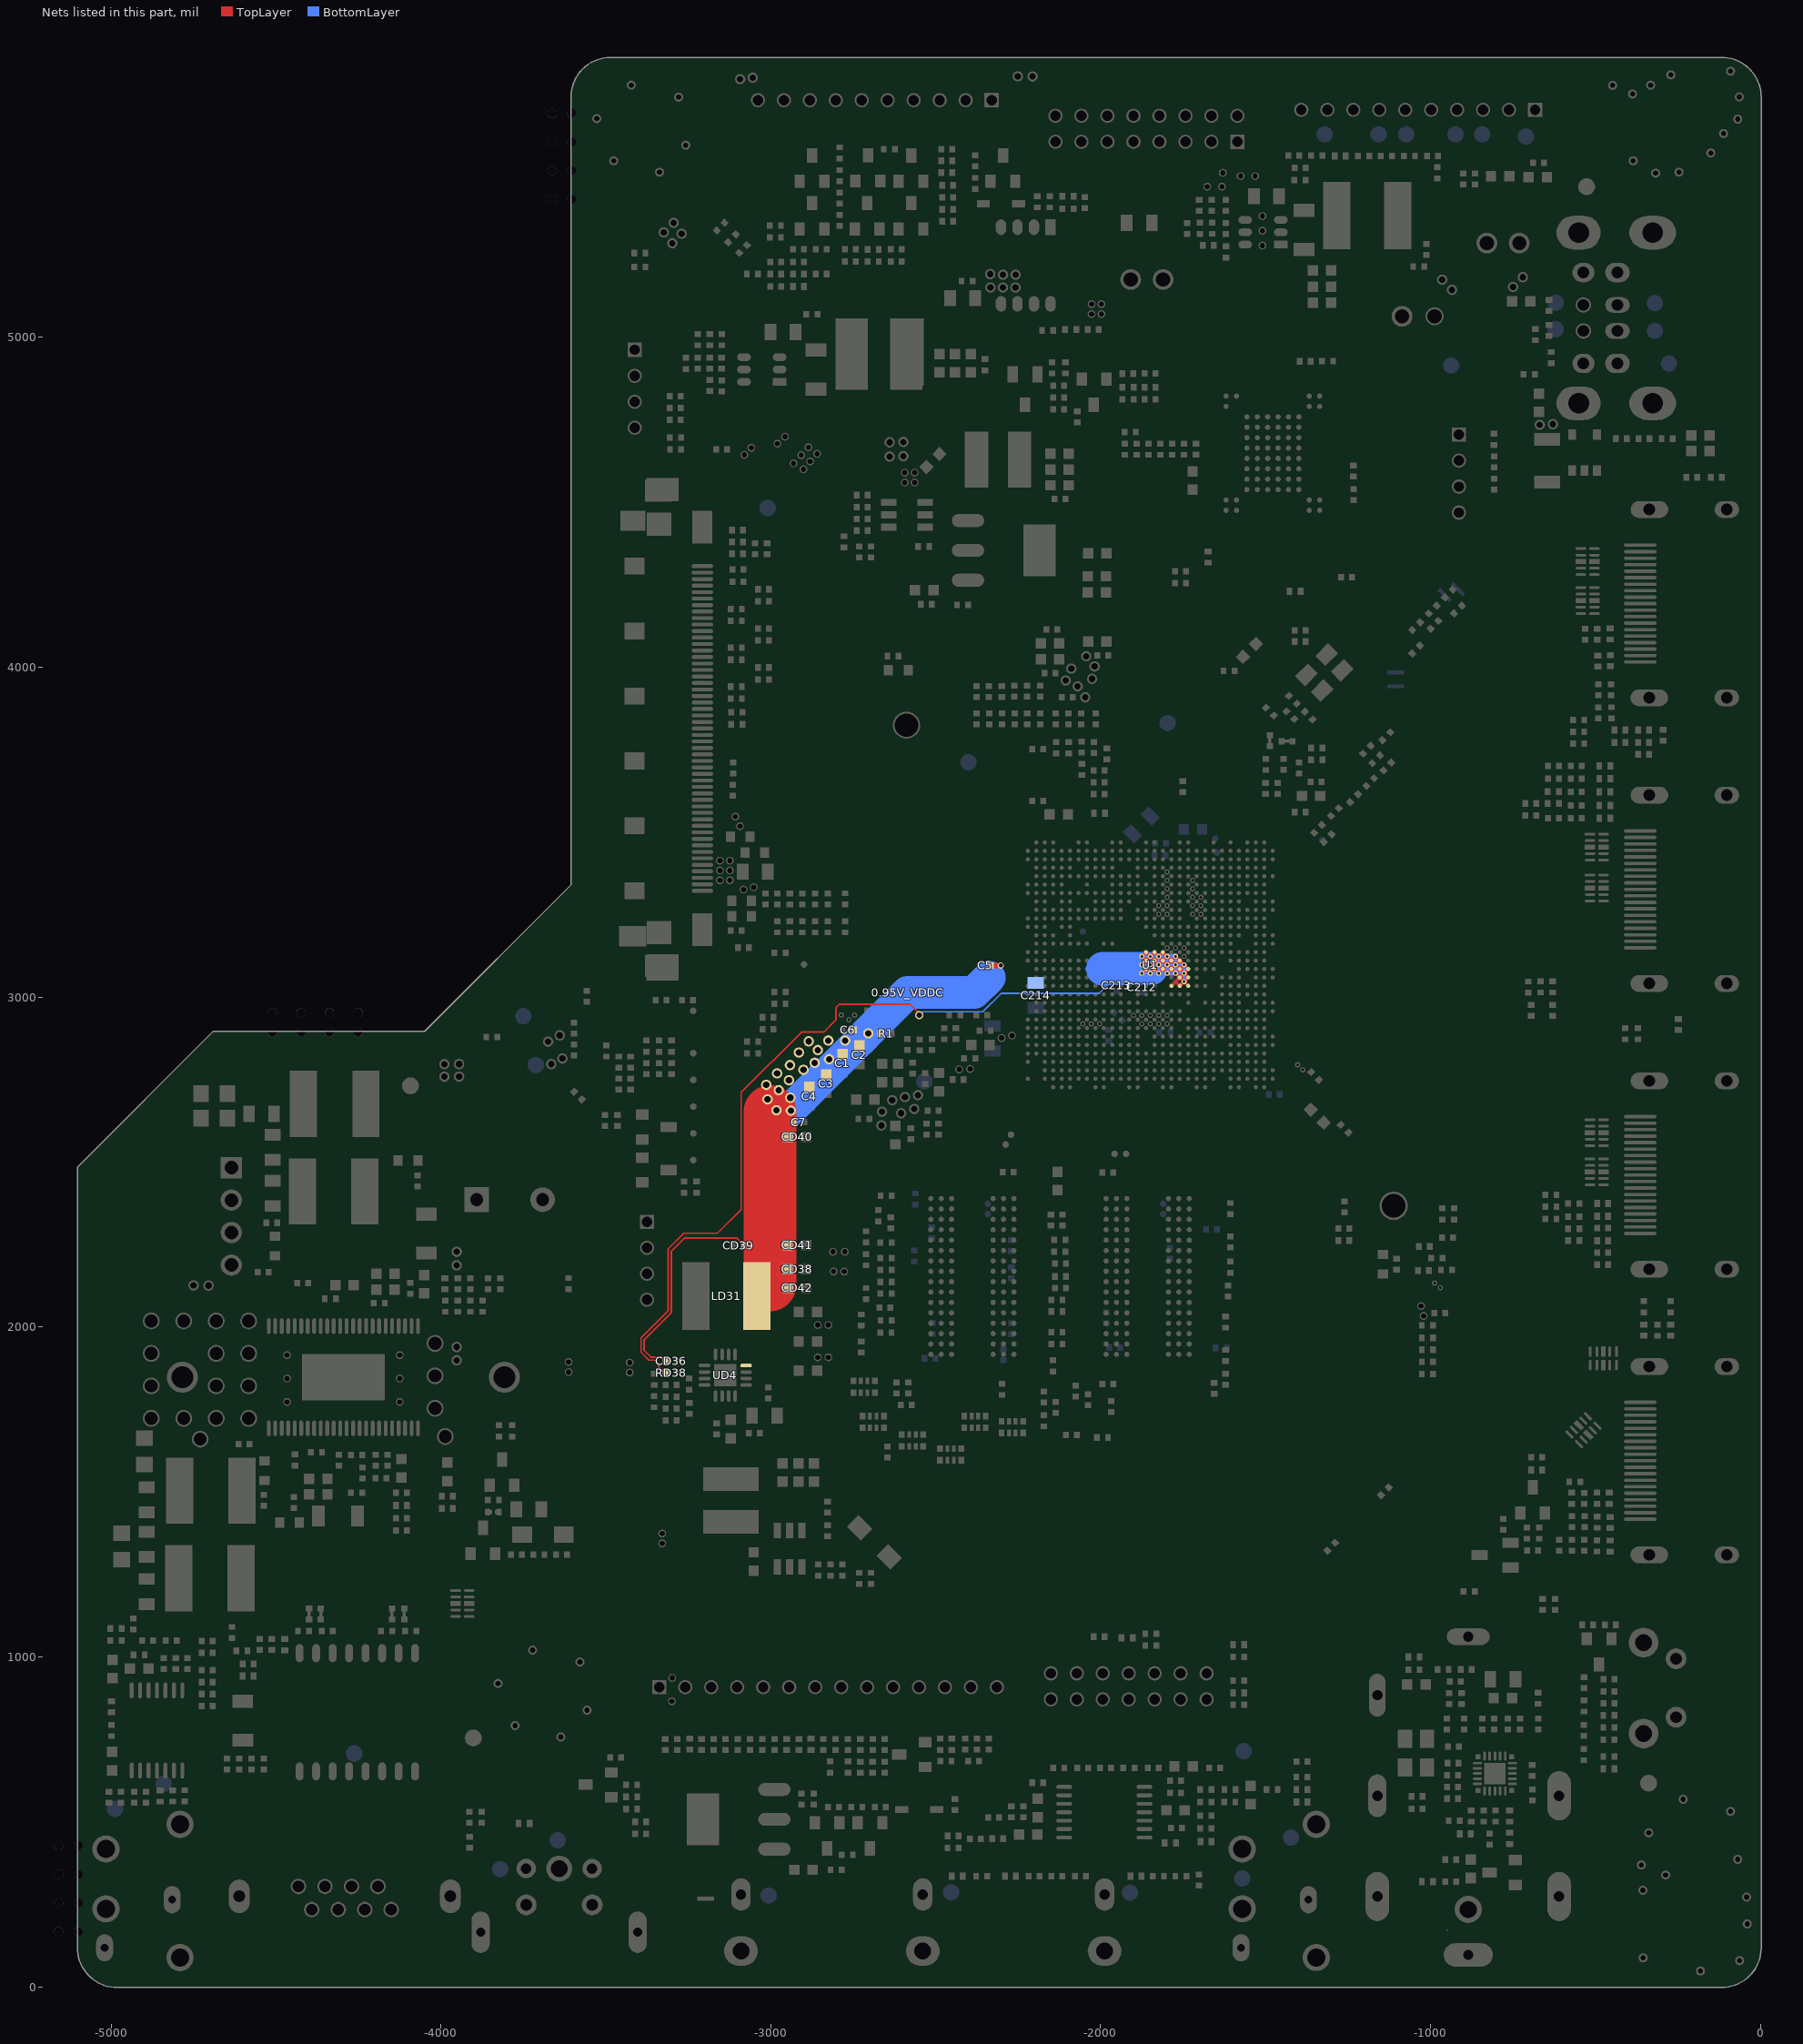
[diagram p0: the nets of this part, all layers, seen from the top]
# Altium PCB MISC86290.PcbDoc (part 7 of 31)
Units mil, origin at the board's own origin, x right, y up, seen from the top; angles counter-clockwise.
Board outline 5104.71 x 5851.49 mil, 2 copper layers (TopLayer, BottomLayer), stack 61.855 mil thick; 1026 components, 667 nets, 4280 pads, 2294 vias.

## Part data (continued)
CA30 CA31: library part 004.003.0000956-D, "Ceramic capacitor,CAP MC,50V,10uF,±10%,X5R,1206,SMD,TP-D"
CA32 CA33 CA34 CA35 CO2: library part 330pF-0402-NPO-±5%-50V-D
CA53 CA56 CO15 CO16: library part 220pF-0402-NPO-±5%-50V-D
CD1 CD13: library part 10uF-1206-X5R-±10%-16V-D
CD2 CD5 CD7 CD32 CD39 CP2 CT10 CT15 CT16 CT17 CT27 CT32 CU14: library part 0.1uF-0402-Y5V-+80%-20%-16V-D
CD6: library part 10pF-0402-NPO-±5%-50V-D
CD15: library part 8pF-0402-NPO-±5%-50V-D
CD23 CD53: library part 004.003.0000527-D, "Ceramic capacitor,CAP MC,50V,18pF,±5%,NPO,0402,SMD,TP-D"
CD34 CM2 CM4 CM16: library part 0.022uF-0402-X7R-±10%-16V-D
CD36 CT24: library part 120pF-0402-NPO-±5%-50V-D
CE1 CE2 CE3 CE4: library part 7pF-0402-NPO-±5%-50V-D
CE5: library part 1000pF-1206-X7R-±20%-2000V-D
CE8: library part 0.01uF-0402-X7R-±10%-16V-D
CH1 CH2 CH4 CH5 CH6 CH11 CH12 CH13 CH14 CH21 CH22 CH23 CH24 CH31 CH32 CH33 CH34: library part 5pF-0402-NPO-±5%-50V-D
CH7: library part 2.2uF-0402-X5R-±20%-6.3V-D
CH15 CH16 CH17 CH18 CK1 CT26: library part 22pF-0402-NPO-±5%-50V-D
CI1 CI3 CI5 CT6 CT7 CT8 CT12 CT14 CT21: library part 56pF-0402-NPO-±5%-50V-D
CI4 CI6: library part 1uF-0402-X5R-±20%-16V-D
CK7 CK8 CM1 CO11 CO12 CO31 CO32 CT1 CT2 CT19 CT20: library part 1000pF-0402-X7R-±10%-50V-D
CM3 CU15 CU16: library part 22uF-0603-X5R-±20%-6.3V-D
CM15 CO18 CO42 CU4 CU11 CU12 CU13: library part 0.1uF-0402-X7R-±10%-16V-D
CN1 CN2 CN3: library part 4PIN-2.0-D-H-G-LD-DHMI
CN16: library part XXX.XXX.0000613-DHMI, "Connector socket,connect jack,10Pin,D2.0,D,L=2.8mm,DIP,CNJST-DHMI"
CN17: library part XXX.XXX.0000646-DHMI, "Connector socket,connect jack,10Pin,D2.0,D,SNAP,L=2.8mm,DIP,CNJST-DHMI"
CN19: library part 10PIN-2.0-D-H-G-带扣-J-DHMI
CNA3: library part XXX.XXX.0000762-DLMI, "Connector socket,connect jack,4Pin,D2.50,L,STEP,Beige,L=2.8mm,DIP,CNJST-DLMI"
CNA4: library part XXX.XXX.0001836-DLMI, "Connector socket,connect jack,4PIN,D2.50,L,SNAP,STEP,Fool-proofing,Nature,L=3.0mm,DIP,AMA-DLMI"
CNA5: library part XXX.XXX.0002239-DHMI, "Gold-plated pin,pin connector,2×7Pin,D,D2.0,L=2.6mm,DIP,LD-DHMI"
CNK2: library part 14PIN-2.0-D-H-G-DHMI-IR&KEY
CNK3: library part 14PIN-2.0-D-H-G-带扣-J-DHMI
CNP2: library part 2×8PIN-2.0-D-H-G-带扣-J-DHMI, "CN-keyed"
CNW1: library part XXX.XXX.0002122, "FPC socket,FPC connector (B),51Pin,D0.5,L,Bottom,lock,SMD,DEREN-D"
CNW2: library part 51PIN-0.5-L-M-下接-翻盖-H=2.7mm-XFE-D, "CN-FFC socket-flip lid"
CNW3: library part PKG-003664/P000081334, "FFC socket,FFC connector,51Pin,D0.5,Bottom,lock,SMD,F05035FA51M1WL,CT-D"
CNW12: library part FI-RE51S-HF-J-R1500-D, "CN-FFC socket-bottom contact"
CO20 CO36: library part 10uF-0603-X5R-±20%-6.3
CO26 CO27: library part 004.003.0000501-D, "Ceramic capacitor,CAP MC,50V,100pF,±5%,NPO,0402,SMD,TP-D"
CT3: library part 10uF-0603-X5R-±20%-10V-D
CT4 CT5: library part 27pF-0402-NPO-±5%-50V-D
CT9 CT23: library part 30pF-0402-NPO-±5%-50V-D
CT25: library part 47pF-0402-NPO-±5%-50V-D
CT28: library part 0.1uF-0805-X7R-±10%-50V-D, "CAP"
CT39 CT40: library part 18pF-0402-NPO-±5%-50V-D
D4 D5 D40 D41 DA1 DA2 DA5 DA6 DG1 DG11 DH15 DI1 DI2 DI3 DK9 DK10 DO1 DO2 DO11 DO12 DO31 DO32 DR1 DR2 DR4 DR5 DT2 DT3: library part AVLC18S02003-D
DA9: library part PMLL4148L-F-D
DD2: library part 5.6V-LL-34-1/2W-D
DE1 DE2 DF5 DF6 DU1 DU2 DW1 DW2: library part AIES12U020R2-D
DH1 DH2 DH3 DH4 DH5 DH11 DH12 DH13 DH14 DH21 DH22 DH23 DH24 DH31 DH32 DH33 DH34 DH35 DH36 DH37: library part "TVS管,DIO ESD,0.4pF,11V,SOD882,SMD,PESD5V0F1BL,NXP-D"
DM11 DR3: library part 1N4148WS-D
DT1: library part BAV99-BR-D
EA1: library part 004.003.0000454-DHMI, "Aluminium electrolytic capacitor,CAP AL,35V,470uF,±20%,RK,P,5.0mm,10×13,DIP,TP,XL-DHMI"
ED1 ED11: library part 470uF-10V-±20%-6.3×11-105℃-黑底白字-编带-F=2.5-XF-DHAI, "Electrolytic"
EP1: library part 004.003.0000158-DHAI, "Aluminium electrolytic capacitor,CAP AL,16V,220uF,±20%,LD,KF,P,2.5mm,6.3×11,DIP,TP,CapXon-DHAI"
FT1 LA10 LA12 RT4: library part FCM1005KF-121T06(120ohm-500mA)-D
FU1: library part NSMD110(1206-1.1A)-D
H1 H2 H3 H4 H5 H6: library part "Location hole-D"
HS1: library part 004.040.0000611-HS, "Heat sink,aluminium alloy,55.0×55.0×10.0mm,black,anodized,THD-HS"
HSA1: library part 27*10*10-HS, "HS-natural colour"
LA1 LA2 LA3 LA4: library part MPIT6045-150M-LF-D
LD1 LD3 LD4: library part SWPA6045S4R7MT-D
LD2: library part MGSD54-6R8M-LF-D
LD21 LD51: library part SLN43T-6R8M-D
LD31: library part 004.004.0000652-D, "Power inductor,Power Inductor,2.2uH,±20%,4.60A,DR6.0×4.5,SMD,MPIT6045-2R2M-LF,Microgate-D"
LF1: library part HCB1005KF-121T20(120ohm-1200mA)-D
LO1 R1 R3 R130 R135 R136 R137 R171 RD3 RD4 RD13 RD14 RD30 RD51 RE6 RF3 RF4 RF5 RF6 RF7 RF8 RG41 RG42 RG43 RG44 RI115 RO3 RO51 RO52 RR18 RT1 RT3 RT7 RT40 RU13 RU14 RU15 RU16 RU17 RW10 RW11 RW389 RW393 RW395: library part 0ohm-0402-±5%-1/16W-D
LO2 LO3: library part 004.004.0000326-D, "Ferrite bead,BEAD,120ohm,0402,500mA,SMD,TP,FCM1005KF-121T06,Tai-tech-D"
LT3 LT4 LT5 LT6 LT7 LT9: library part SDCL1005CR33JTDF-D
LT10: library part 680ohm-0402-±5%-1/16W-D
LU11: library part HCB1608KF-121T20(120ohm-2000mA)-D
M1 M2 M3 M4 M5 M6: library part MARK-D
MAC: library part Barcode
NC/ESD: library part ESD-T
P1(用于U1上): library part 0.05g-导热硅脂, "Thermal grease"
QA2: library part 3CG3906M-D, "Q-PNP-#-#-#"
QA3 QG1 QG2 QG11 QG12 QG30 QG31 QK1 QO21 QR3: library part LMBT3904LT1G-D-NPN, "Q-NPN-#-#-#"
QM1: library part WPM3407C-3/TR-D
QM2: library part AO4459-D
QM4 QM11 QR4: library part KMBT3904-D
QR1 QR2: library part LMBT3906LT1G-D-PNP
QW1 QW2: library part 004.007.0000056-D, "MOSFET,NMOS,0.3A,60V,3.3ohm@ID=0.3A@VGS=4.5V,SOT-23,ME2N7002E,MATSUKI-D"
R4 R5 R6 R7 R8 R9 R10 R11 R12 R13 R14 R15 R16 R17 R18 R19 R20 R21 R22 R23 R24 R25 R26 R27 RD21 RD24 RD52: library part 004.002.0000689-D, "Thick-film resistor,RES,1/16W,4.7Kohm,±5%,0402,SMD-D"
R30 R31 R138 R139 R151 R152 R153 RA11 RA20 RG2 RG30 RG31 RK1 RK28 RK30 RM1 RM2 RM11 RM13 RM15 RO20 RO22 RO23 RO26 RO27 RO28 RO29 RO30 RO43 RO44 RO45 RO46 RO47 RP5 RR3 RR9 RR13 RR15 RR16 RT5 RT6 RU3 RU6 RU11 RU12 RU18 RW4 RW251 RW252 RW405 RW406 RW407 RW408 RW409 RW410 RW412 RW413 RW414 RW415 RW416 RW417: library part 4K7ohm-0402-±5%-1/16W-D
R39: library part 004.002.0000721-D, "Thick-film resistor,RES,1/16W,68ohm,±5%,0402,SMD-D"
R41 R54 R55 R58 R59 R60 R61: library part 004.002.0000728-D, "Thick-film resistor,RES,1/16W,75ohm,±5%,0402,SMD-D"
R42 R208 RD2: library part 1Mohm-0402-±5%-1/16W-D
R44 R120 RF1: library part 004.002.0000572-D, "Thick-film resistor,RES,1/16W,1Kohm,±5%,0402,SMD-D"
R45 R62 R63 R107 R108 R121 R123: library part 004.002.0000577-D, "Thick-film resistor,RES,1/16W,10Kohm,±5%,0402,SMD-D"
R46 R47: library part 004.002.0000583-D, "Thick-film resistor,RES,1/16W,11Kohm,±1%,0402,SMD-D"
R48 R49 R64 R100: library part 004.002.0000636-D, "Thick-film resistor,RES,1/16W,240ohm,±1%,0402,SMD-D"
R50 R51 R52 R53 R56 R57: library part 004.002.0000626-D, "Thick-film resistor,RES,1/16W,22ohm,±5%,0402,SMD-D"
R65 R66 R67 R101 R102 R103 R104 R118: library part 004.002.0000575-D, "Thick-film resistor,RES,1/16W,10Kohm,±1%,0402,SMD-D"
R72 R73 R140 R141 RA9 RH37 RH38 RR5 RR8 RT2 RT8 RT9 RW5: library part 100ohm-0402-±5%-1/16W-D
R105 R106: library part 004.002.0000447-D, "Thick-film resistor,RES,1/16W,56ohm,±1%,0402,SMD-D"
R122 R124: library part 004.002.0000630-D, "Thick-film resistor,RES,1/16W,2.2Kohm,±5%,0402,SMD-D"
R125 R126 R127 R128 R129 RH1 RH4 RH11 RH12 RH21 RH22 RH31 RH32: library part 004.002.0000658-D, "Thick-film resistor,RES,1/16W,33ohm,±5%,0402,SMD-D"
R143 R144 R145 R206 R207 RA21 RA23 RG1 RG7 RG12 RG17 RG37 RG38 RK2 RK10 RK26 RK33 RK42 RO24 RO25 RO39 RO40 RR1 RT10 RT12: library part 1Kohm-0402-±5%-1/16W-D
R146 R147 R148 R149 R150 RG3 RG13 RG39 RI1 RR10 RR11 RR14 RW26 RW73 RW421: library part 33ohm-0402-±5%-1/16W-D
R200 R201 R202 R203 R204 R205 RD1 RD11 RD12 RG32 RG33 RO13 RO14 RO33 RO34 RO55 RO56 RR19: library part 100Kohm-0402-±5%-1/16W-D
RA1 RA2 RA3 RA4 RH5 RH6 RH15 RH16 RH25 RH26 RH35 RH36 RK23: library part 22ohm-0402-±5%-1/16W-D
RA5 RA7 RA34 RG6 RG8 RG11 RG16 RG18 RG34 RG36 RH2 RH3 RH13 RH14 RH23 RH24 RH33 RH34 RI3 RI6 RK15 RM12 RP1 RR2 RR6 RR7 RR17 RU5 RU9 RU10 RW1 RW8 RW9: library part 10Kohm-0402-±5%-1/16W-D
RA6 RA8 RA12 RA14: library part 470ohm-0402-±5%-1/16W-D
RA15: library part 18Kohm-0402-±1%-1/16W-D
RA16 RA17 RA18 RA19: library part 18ohm-0603-±5%-1/10W-D
RA22: library part 8K2ohm-0402-±5%-1/16W-D
RA24 RA26 RK13 RO11 RO12 RO31 RO32: library part 33Kohm-0402-±5%-1/16W-D
RA30 RA31 RA32 RA33: library part 300ohm-2500mA-0805-D
RD5: library part 30Kohm-0402-±5%-1/16W-D
RD6: library part 3K3ohm-0402-±5%-1/16W-D
RD15 RD38: library part 60K4ohm-0402-±1%-1/16W-D
RD16: library part 10K5ohm-0402-±1%-1/16W-D
RD22 RD53 RD60: library part 004.002.0000718-D, "Thick-film resistor,RES,1/16W,6.2Kohm,±1%,0402,SMD-D"
RD23 RD54 RD55 RD57 RD59: library part 004.002.0000622-D, "Thick-film resistor,RES,1/16W,20Kohm,±1%,0402,SMD-D"
RD32 RD34 RD36: library part 113Kohm-0402-±1%-1/16W-D
RD33 RD35 RD37: library part 47Kohm-0402-±1%-1/16W-D
RD58: library part 004.002.0000558-D, "Thick-film resistor,RES,1/16W,0ohm,±5%,0402,SMD-D"
RE1 RE2 RE3 RE4: library part 75ohm-0402-±1%-1/16W-D
RE20 RE21 RE22 RE23 RT11 RT13: library part 0ohm-0402-PCB-D, "0ohm-0402-PCB-D"
RF2: library part 004.002.0000675-D, "Thick-film resistor,RES,1/16W,3.9Kohm,±1%,0402,SMD-D"
RF56: library part 004.002.0000757-D, "Thick-film resistor,RES,1/16W,120Kohm,±1%,0402,SMD-D"
RFT1: library part XXX.XXX.0002536, "RF shield can,RF SHLED,Single,H,F,T14.5,CH6.3,whole,25.0×14.5×10.0mm,DIP,LHD-DLMI"
RG4 RG5 RG14 RG15 RG35 RG40 RP8 RR4: library part 2K2ohm-0402-±5%-1/16W-D
RH17 RO1: library part 200ohm-0402-±5%-1/16W-D
RI2 RO2: library part 75ohm-0402-±5%-1/16W-D
RI4 RI5 RO19 RO21 RO41 RO42: library part 12Kohm-0402-±5%-1/16W-D
RI116 RO17 RO18 RO35 RO36: library part GND
RK14: library part 510ohm-0402-±5%-1/16W-D
RK24 RK34: library part 4K7ohm-0402-±1%-1/16W-D
RK27 RK32 RK35 RK36 RK37 RK38 RK40 RK41: library part 1K5ohm-0402-±5%-1/16W-D
RK29 RK31: library part 12Kohm-0402-±1%-1/16W-D
RM3 RM4 RM14 RO57 RO58: library part 47Kohm-0402-±5%-1/16W-D
RO15 RO16 RO37 RO38 RU1 RU2 RU7 RU8: library part 5R1ohm-0402-±5%-1/16W-D
RO53 RO54: library part 004.002.0000624-D, "Thick-film resistor,RES,1/16W,200Kohm,±5%,0402,SMD-D"
RP11 RP12 RP13 RP14 RP15 RP16: library part 4*56ohm-0402-±5%-1/16W-D
SK1: library part "轻触开关,Tact Switch,160±50gf,7.0×10.3×7.0mm,DIP,KFC-A06-E-4-7.5/4(R),YK-DLMI"
SKT1: library part SG-BGA-6367-TEST, "SG-BGA-6367 test socket"
U1: library part 004.016.0001110-D, "TV main chip,IC Main Chip,MSDURN1801-Z1,64bit,Multi-Core,BGA758,SMD,Mstar-D"
U2 U3: library part 004.011.0000261-D, "DDR chip,DDR3,1866M,4Gb(256M×16bit),FBGA96,SMD,K4B4G1646E-BCMA,Samsung-D"
UA1: library part PKG-002027/P000038588, "Audio amplifier,IC Audio AMP,Class D,2×20W@18.0V@8ohm,HTSSOP48,SMD,TAS5751MDCAR,TI-D"
UA2 UA3: library part APA2171-D
UD1: library part MP1470GJ-Z-D
UD2: library part MP1471AGJ-Z-D
UD3 UD5: library part 004.010.0000967-D, "DC-DC chip,IC DCDC,Syn,2A,5.5V,1.5MHz,SOT23-6,SMD,TLV62569PDDCR,TI-D"
UD4: library part 004.010.0000812, "DC-DC chip,IC DC-DC,Syn,4A,5.5V,1.4MHz,VQFN-16,SMD,TLV62095RGTR,TI-D"
UE1: library part H16101MC-D
UE2 UH1 UH2 UH11 UH12 UH21 UH22 UH31 UH32: library part ULC0524P-D, "RCLAMP0524J"
UF1: library part PKG-003578/P000079162, "NAND FLASH chip,512MB,4Gb,TC58NVG2S0HBAI4,TOSHIBA-D"
UH3: library part AP2171WG-7-D
UL1: library part LC1117CLTR33-D
UL2: library part LC1117CLTRAD-D
UR1: library part SGM809-SXN3-D
UT2: library part "硅高频头,IC Si Tuner,QFN-24,SMD,SI2159-A10-GMR,Silicon Labs-D"
Y1 YT2: library part 16.000MHz±20PPM-10PF-SMD3225-D

## Free pads (board coordinates)
  round 27.56 hole 27.56 unplated: 0(-5158.73,167.32) 0(-5158.73,253.94) 0(-5158.73,340.55) 0(-5158.73,427.16) 0(-5099.68,167.32) 0(-5099.68,253.94) 0(-5099.68,340.55) 0(-5099.68,427.16) 0(-4511.06,2893.7) 0(-4511.06,2952.76) 0(-4424.44,2893.7) 0(-4424.44,2952.76) 0(-4337.83,2893.7) 0(-4337.83,2952.76) 0(-4251.21,2952.76) 0(-4251.21,2893.7) 0(-3662.67,5419.29) 0(-3662.67,5505.9) 0(-3662.67,5592.52) 0(-3662.67,5679.13) 0(-3603.61,5419.29) 0(-3603.61,5505.9) 0(-3603.61,5592.52) 0(-3603.61,5679.13)
  round 157.48 on Keep-Out: 0(-511.81,5649.61)
  oval 196.85x157.48 on Keep-Out: 0(-452.76,196.85)
  round 51.18 hole 39.37 paste-15.75 mask-15.75: VIA5(-4878.28,1723) VIA5(-4878.28,1821.43) VIA5(-4878.28,1919.85) VIA5(-4878.28,2018.27) VIA5(-4779.85,1723) VIA5(-4779.85,2018.27) VIA5(-4730,1660) VIA5(-4681.42,1723) VIA5(-4681.42,1821.43) VIA5(-4681.42,1919.85) VIA5(-4681.42,2018.27) VIA5(-4583,1723) VIA5(-4583,1821.43) VIA5(-4583,1919.85) VIA5(-4583,2018.27) VIA5(-4018,1753.43) VIA5(-4018,1851.85) VIA5(-4018,1950.27) VIA5(-3987,1668)
  round 31.5 hole 19.68 paste-15.75 mask-15.75: VIA5(-4750,2126) VIA5(-4704.69,2125.6) VIA5(-3989.5,2758.79) VIA5(-3989.5,2796.79) VIA5(-3952.5,1899) VIA5(-3952.5,1939.22) VIA5(-3952.5,2187) VIA5(-3952,2228) VIA5(-3945,2759) VIA5(-3945,2797) VIA5(-3675,2865) VIA5(-3666,2797) VIA5(-3640,2884) VIA5(-3631.84,2813.88) VIA5(-3324.5,5318.5) VIA5(-3298.5,5285.5) VIA5(-3294.5,5347.5) VIA5(-3270.5,5314.5) VIA5(-3093.07,5782.96) VIA5(-3054.69,5787.5) VIA5(-3014,2734) VIA5(-3010,2690) VIA5(-2983,2657) VIA5(-2981,2769) VIA5(-2976,2718) VIA5(-2945,2748) VIA5(-2942,2794) VIA5(-2941,2695) VIA5(-2939.25,2656) VIA5(-2915,2832) VIA5(-2901,2779.5) VIA5(-2885,2866) VIA5(-2867,2801) VIA5(-2857.5,2839.5) VIA5(-2825.5,2868.5) VIA5(-2823.5,2812) VIA5(-2774.5,2868.5) VIA5(-2704.5,2890) VIA5(-2665,2611) VIA5(-2663,2652.5) VIA5(-2640,4639) VIA5(-2640,4682) VIA5(-2632,2687.5) VIA5(-2605,2648) VIA5(-2598,4640) VIA5(-2598,4683) VIA5(-2593.5,2697) VIA5(-2565.5,2661) VIA5(-2554,2703.03) VIA5(-2335,5192) VIA5(-2334.35,5151.26) VIA5(-2296.35,5151.26) VIA5(-2296,5190) VIA5(-2258.35,5151.26) VIA5(-2258,5190) VIA5(-2251.5,5791.5) VIA5(-2206.5,5791) VIA5(-2106,3960) VIA5(-2089,3996) VIA5(-2070,3942) VIA5(-2047,3909) VIA5(-2044,4033.5) VIA5(-2026,3965) VIA5(-2018.5,4002.5) VIA5(-965,5175) VIA5(-935,5144) VIA5(-750,5153) VIA5(-720.3,5182.7) VIA5(-669,4735) VIA5(-629,4737)
  round 23.62 hole 15.75 paste-15.75 mask-15.75: VIA5(-4466.68,1772.94) VIA5(-4466.68,1843.81) VIA5(-4466.68,1914.68) VIA5(-4124.82,1772.94) VIA5(-4124.82,1843.81) VIA5(-4124.82,1914.68) VIA5(-3613,1863) VIA5(-3613,1894) VIA5(-3428,1862) VIA5(-3428,1892) VIA5(-3329.25,1344) VIA5(-3329.25,1374) VIA5(-3300,865) VIA5(-3298.97,936) VIA5(-3154.25,3354) VIA5(-3154.25,3384) VIA5(-3154.25,3414) VIA5(-3124.25,3354) VIA5(-3124.25,3384) VIA5(-3124.25,3414) VIA5(-3107.5,3547.5) VIA5(-3093.5,3518.5) VIA5(-3082.5,3326) VIA5(-3080.25,4644) VIA5(-3059.03,4665.21) VIA5(-3052,3333) VIA5(-2980.21,4678.2) VIA5(-2957,4699) VIA5(-2931,4618) VIA5(-2908,4643) VIA5(-2901,4600) VIA5(-2886,4667) VIA5(-2881,4624) VIA5(-2860,4647) VIA5(-2857.72,1908.03) VIA5(-2857.72,2006.03) VIA5(-2825.72,1908.03) VIA5(-2825.72,2006.03) VIA5(-2811.72,2228.03) VIA5(-2809.72,2168.03) VIA5(-2777.72,2168.03) VIA5(-2775.72,2228.03) VIA5(-2594,4560) VIA5(-2594,4590) VIA5(-2564,4560) VIA5(-2564,4590) VIA5(-2027.75,5070.84) VIA5(-2027.75,5100.84) VIA5(-1997.75,5070.84) VIA5(-1997.75,5100.84) VIA5(-1677.18,5457.24) VIA5(-1632.47,5457.24) VIA5(-1630,5499) VIA5(-1576.18,5489.2) VIA5(-1531.47,5489.2) VIA5(-1509.77,5278.53) VIA5(-1509.77,5323.24) VIA5(-1509.77,5367.94) VIA5(-1029,2063.5) VIA5(-1021,2033.5)
  round 15.75 hole 7.87 paste-15.75 mask-15.75: VIA5(-2786.56,2945.94) VIA5(-2763.06,2931.44) VIA5(-2746.06,2945.44) VIA5(-2054.45,2918.9) VIA5(-2028.86,2918.9) VIA5(-2003.27,2918.9) VIA5(-1900.91,2944.49) VIA5(-1875.32,2918.9) VIA5(-1875.32,2944.49) VIA5(-1875.32,3072.44) VIA5(-1875.32,3098.03) VIA5(-1875.32,3123.62) VIA5(-1849.72,3098.03) VIA5(-1849.72,2918.9) VIA5(-1849.72,2944.49) VIA5(-1849.72,3072.44) VIA5(-1849.72,3123.62) VIA5(-1824.13,2918.9) VIA5(-1824.13,2944.49) VIA5(-1824.13,3072.44) VIA5(-1824.13,3098.03) VIA5(-1824.13,3123.62) VIA5(-1824.13,3251.57) VIA5(-1824.13,3277.17) VIA5(-1798.54,3251.57) VIA5(-1798.54,2918.9) VIA5(-1798.54,2944.49) VIA5(-1798.54,3072.44) VIA5(-1798.54,3123.62) VIA5(-1798.54,3149.21) VIA5(-1798.54,3277.17) VIA5(-1798.54,3302.76) VIA5(-1798.54,3328.35) VIA5(-1798.54,3353.94) VIA5(-1798.54,3379.53) VIA5(-1798.54,3098.03) VIA5(-1772.95,3072.44) VIA5(-1772.95,3098.03) VIA5(-1772.95,3123.62) VIA5(-1772.95,3149.21) VIA5(-1747.36,3046.85) VIA5(-1747.36,3072.44) VIA5(-1747.36,3098.03) VIA5(-1747.36,3123.62) VIA5(-1747.36,3149.21) VIA5(-1721.77,3251.57) VIA5(-1721.77,3277.17) VIA5(-1721.77,3302.76) VIA5(-1721.77,3328.35) VIA5(-1721.77,3353.94) VIA5(-1696.18,3251.57) VIA5(-1696.18,3277.17) VIA5(-1696.18,3302.76) VIA5(-1403.01,2795.01) VIA5(-1387.45,2779.45) VIA5(-988,2133) VIA5(-970.44,2119)
  round 24 / inner round 60 / far side round 24 hole 16: VIA5(-2429,2781) VIA5(-2396.1,2782.4) VIA5(-2300.6,2876.14) VIA5(-2269.02,2883.46)

## Via types
v1: diameter 19.68, hole 11.81, TopLayer to BottomLayer, tented both sides, 1189 vias
v2: diameter 19.68/19.68 (per signal layer), hole 11.81, TopLayer to BottomLayer, tented both sides, 366 vias
v3: diameter 15.75, hole 7.87, TopLayer to BottomLayer, tented both sides, 348 vias
v4: diameter 23.62, hole 15.75, TopLayer to BottomLayer, tented both sides, 309 vias
v5: diameter 15.75/15.75 (per signal layer), hole 7.87, TopLayer to BottomLayer, tented both sides, 59 vias
v6: diameter 24/24 (per signal layer), hole 16, TopLayer to BottomLayer, tented both sides, 23 vias

## Nets (pads, with @x,y where several pads share a name; then routed paths per layer and width w, separated by ;. In a path a pad name is that pad's centre, name@x,y a point inside that pad or via, vN(x,y) a via of type N, cw(c..) or ccw(c..) an arc to the next point about the centre after c; other vN are vias at no path point)
0.95V_VDDC: 0.95V_VDDC.1 C1.2 C2.2 C3.2 C4.2 C5.1 C6.1 C7.1 C212.1 C213.1 C214.1 CD36.2 CD38.2 CD39.2 CD40.2 CD41.2 CD42.2 LD31.2 pad.VIA5@-1747.36,3046.85 pad.VIA5@-1747.36,3072.44 pad.VIA5@-1747.36,3098.03 pad.VIA5@-1772.95,3072.44 pad.VIA5@-1772.95,3098.03 pad.VIA5@-1772.95,3123.62 pad.VIA5@-1798.54,3072.44 pad.VIA5@-1798.54,3098.03 pad.VIA5@-1798.54,3123.62 pad.VIA5@-1824.13,3072.44 pad.VIA5@-1824.13,3098.03 pad.VIA5@-1824.13,3123.62 pad.VIA5@-1849.72,3072.44 pad.VIA5@-1849.72,3098.03 pad.VIA5@-1849.72,3123.62 pad.VIA5@-1875.32,3072.44 pad.VIA5@-1875.32,3098.03 pad.VIA5@-1875.32,3123.62 pad.VIA5@-2704.5,2890 pad.VIA5@-2774.5,2868.5 pad.VIA5@-2823.5,2812 pad.VIA5@-2825.5,2868.5 pad.VIA5@-2857.5,2839.5 pad.VIA5@-2867,2801 pad.VIA5@-2885,2866 pad.VIA5@-2901,2779.5 pad.VIA5@-2915,2832 pad.VIA5@-2939.25,2656 pad.VIA5@-2941,2695 pad.VIA5@-2942,2794 pad.VIA5@-2945,2748 pad.VIA5@-2976,2718 pad.VIA5@-2981,2769 pad.VIA5@-2983,2657 pad.VIA5@-3010,2690 pad.VIA5@-3014,2734 R1.1 RD38.2 U1.N11 U1.N12 U1.N13 U1.P11 U1.P12 U1.R11 U1.R12 U1.R13 U1.R14 U1.R15 U1.R16 U1.T12 U1.T13 U1.T14 U1.T15 U1.T16 U1.U14 U1.U15 U1.U16 UD4.16 | length 5996.8
  TopLayer w5: RD38.2@-3319.23,1867.76 RD38.2@-3319.23,1861 -3321.5,1861 -3340.16,1879.66 -3340.16,1888.68 -3350.99,1899.51 -3369.51,1899.51 -3393.5,1923.5 -3393.5,1966.5 -3311.5,2048.5 -3311.5,2236.5 -3264,2284 -3162.25,2284 -3089.91,2356.35 -3089.91,2711.01 -2906.91,2894 -2839.67,2894 -2802.66,2931.01 -2802.66,2968.2 -2792.86,2978 -2577.61,2978 -2549.97,2950.36 v6(-2549.97,2945.03) ; CD36.2@-3319.23,1897 -3330.89,1908.66 -3363.57,1908.66 -3384,1929.09 -3384,1961.5 -3301.5,2044 -3301.5,2230.5 -3262.5,2269.5 -3102.5,2269.5 -3081.52,2248.52 CD39.2@-3081.52,2247
  TopLayer w10: pad.VIA5@-1875.32,3072.44 U1.R16@-1862.52,3085.24 ; U1.N13@-1785.75,3034.06 -1772.95,3046.85 ; U1.N11@-1734.57,3034.06 pad.VIA5@-1747.36,3046.85 ; U1.R16@-1862.52,3085.24 pad.VIA5@-1849.72,3072.44 U1.R15@-1836.93,3085.24 ; U1.R16@-1862.52,3085.24 pad.VIA5@-1875.32,3098.03 U1.T16@-1862.52,3110.83 ; U1.R16@-1862.52,3085.24 pad.VIA5@-1849.72,3098.03 ; U1.T16@-1862.52,3110.83 pad.VIA5@-1849.72,3123.62 ; U1.T16@-1862.52,3110.83 pad.VIA5@-1875.32,3123.62 U1.U16@-1862.52,3136.42 pad.VIA5@-1849.72,3123.62 ; U1.T16@-1862.52,3110.83 pad.VIA5@-1849.72,3098.03 ; pad.VIA5@-1849.72,3098.03 U1.R15@-1836.93,3085.24 ; pad.VIA5@-1849.72,3098.03 U1.T15@-1836.93,3110.83 ; pad.VIA5@-1849.72,3123.62 U1.U15@-1836.93,3136.42 pad.VIA5@-1824.13,3123.62 ; pad.VIA5@-1849.72,3123.62 U1.T15@-1836.93,3110.83 ; U1.R15@-1836.93,3085.24 pad.VIA5@-1824.13,3072.44 U1.R14@-1811.34,3085.24 ; U1.R15@-1836.93,3085.24 pad.VIA5@-1824.13,3098.03 ; U1.T15@-1836.93,3110.83 pad.VIA5@-1824.13,3098.03 ; U1.T15@-1836.93,3110.83 pad.VIA5@-1824.13,3123.62 ; pad.VIA5@-1824.13,3098.03 U1.T14@-1811.34,3110.83 ; pad.VIA5@-1824.13,3098.03 U1.R14@-1811.34,3085.24 ; pad.VIA5@-1824.13,3123.62 U1.T14@-1811.34,3110.83 ; pad.VIA5@-1824.13,3123.62 U1.U14@-1811.34,3136.42 pad.VIA5@-1798.54,3123.62 ; U1.R14@-1811.34,3085.24 pad.VIA5@-1798.54,3072.44 U1.R13@-1785.75,3085.24 ; U1.R14@-1811.34,3085.24 pad.VIA5@-1798.54,3098.03 ; U1.T14@-1811.34,3110.83 pad.VIA5@-1798.54,3098.03 ; U1.T14@-1811.34,3110.83 pad.VIA5@-1798.54,3123.62 ; pad.VIA5@-1798.54,3098.03 U1.R13@-1785.75,3085.24 ; pad.VIA5@-1798.54,3098.03 U1.T13@-1785.75,3110.83 ; pad.VIA5@-1798.54,3123.62 U1.T13@-1785.75,3110.83 ; U1.R13@-1785.75,3085.24 pad.VIA5@-1772.95,3072.44 ; U1.R13@-1785.75,3085.24 pad.VIA5@-1772.95,3098.03 ; U1.T13@-1785.75,3110.83 pad.VIA5@-1772.95,3123.62 U1.T12@-1760.16,3110.83 ; U1.T13@-1785.75,3110.83 pad.VIA5@-1772.95,3098.03 ; -1772.95,3046.85 U1.P12@-1760.16,3059.65 ; -1772.95,3046.85 U1.N12@-1760.16,3034.06 pad.VIA5@-1747.36,3046.85 ; pad.VIA5@-1772.95,3072.44 U1.R12@-1760.16,3085.24 ; pad.VIA5@-1772.95,3072.44 U1.P12@-1760.16,3059.65 ; pad.VIA5@-1772.95,3098.03 U1.R12@-1760.16,3085.24 ; pad.VIA5@-1772.95,3098.03 U1.T12@-1760.16,3110.83 ; U1.P12@-1760.16,3059.65 pad.VIA5@-1747.36,3072.44 ; U1.P12@-1760.16,3059.65 pad.VIA5@-1747.36,3046.85 ; U1.R12@-1760.16,3085.24 pad.VIA5@-1747.36,3072.44 ; U1.R12@-1760.16,3085.24 pad.VIA5@-1747.36,3098.03 ; U1.T12@-1760.16,3110.83 pad.VIA5@-1747.36,3098.03 ; pad.VIA5@-1747.36,3046.85 U1.P11@-1734.57,3059.65 pad.VIA5@-1747.36,3072.44 ; pad.VIA5@-1747.36,3072.44 U1.R11@-1734.57,3085.24 pad.VIA5@-1747.36,3098.03
  TopLayer w17: C5.1@-2332.27,3096 v1(-2303,3096)
  TopLayer w35: -2950.97,2554.03 -2950.97,2618 -2950.97,2626.03
  TopLayer w160: LD31.2@-3002.25,2127 -3002.25,2618 -3002.25,2653
  BottomLayer w5: v6(-2549.97,2945.03) -2539.5,2955.5 -2357.26,2955.5 -2301.22,3011.53 -2004.47,3011.53 -1975,3041
  BottomLayer w15.75: pad.VIA5@-1849.72,3123.62 pad.VIA5@-1798.54,3123.62 pad.VIA5@-1772.95,3123.62 -1772.95,3115.75 -1764.09,3106.89 -1755.24,3098.03 pad.VIA5@-1747.36,3098.03 pad.VIA5@-1747.36,3072.44 ; pad.VIA5@-1824.13,3072.44 pad.VIA5@-1798.54,3072.44 pad.VIA5@-1772.95,3072.44 ; pad.VIA5@-1747.36,3046.85 -1747.36,3056.69 ; pad.VIA5@-1772.95,3072.44 pad.VIA5@-1772.95,3098.03 pad.VIA5@-1747.36,3072.44 ; pad.VIA5@-1772.95,3072.44 -1763.11,3072.44 ; -1763.11,3072.44 -1755.24,3064.57 -1747.36,3056.69 ; -1763.11,3072.44 pad.VIA5@-1747.36,3072.44 ; -1747.36,3056.69 pad.VIA5@-1747.36,3072.44
  BottomLayer w59.06: -1847.22,3086.53 -1842.72,3091.03 -1835.72,3098.03 pad.VIA5@-1824.13,3098.03 pad.VIA5@-1798.54,3098.03
  BottomLayer w100: pad.VIA5@-2943.5,2655.5 -2728.89,2870.11 ; -2717.97,2881.03 0.95V_VDDC.1@-2585,3014 -2383.76,3014 -2337.72,3060.03 ; -1993.52,3084.56 -1993.52,3086.53 -1849.72,3086.53 -1847.22,3086.53